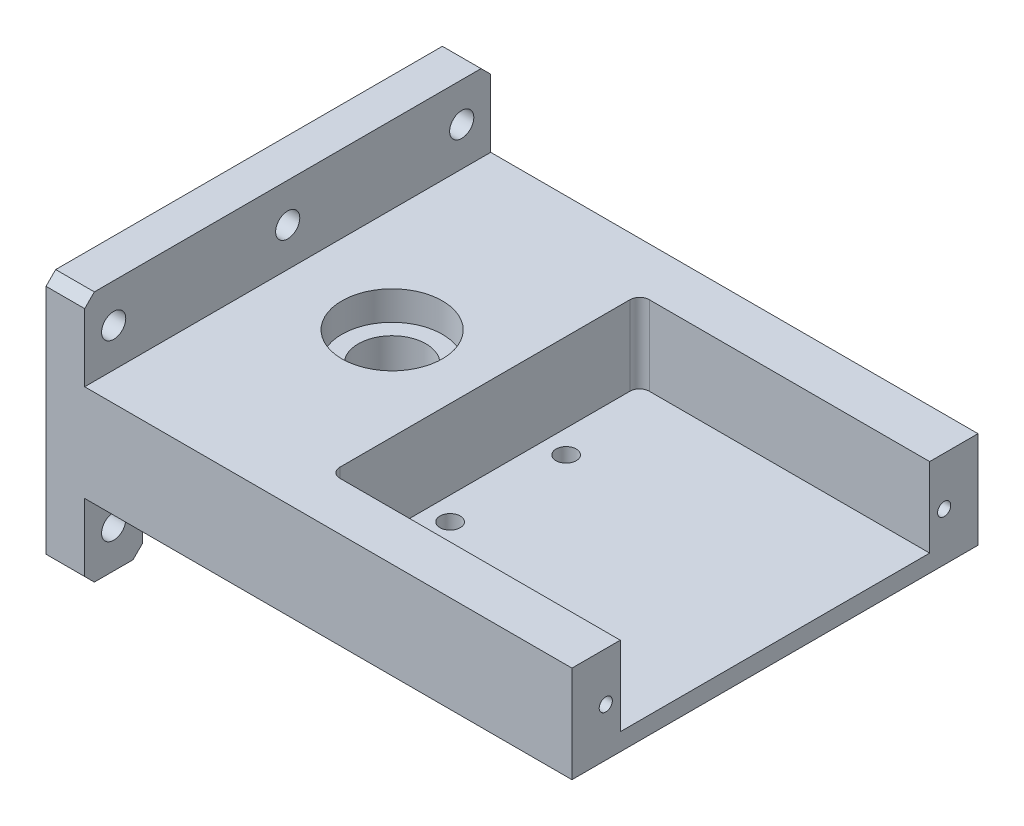
from build123d import *

# Parameters (mm, degrees)
SKETCH_1_W                = 210
SKETCH_1_H                = 130
EXTRUDE_1_DEPTH           = 20
SKETCH_2_W                = 210
SKETCH_2_H                = 50
EXTRUDE_2_DEPTH           = 252
SKETCH_3_R                = 26
CUT_EXTRUDE_1_DEPTH       = 15
SKETCH_4_R                = 17.5
CUT_EXTRUDE_2_DEPTH       = 302.054812285
SKETCH_5_W                = 160
SKETCH_5_H                = 41
CUT_EXTRUDE_3_DEPTH       = 150
HOLE_WIZARD_M8_1_D        = 6.8
HOLE_WIZARD_M8_1_DEPTH    = 19.75
HOLE_WIZARD_M8_1_TIP      = 2.042926105
HOLE_WIZARD_10_5_10_5_1_D = 10.5
SKETCH_10_W               = 150
SKETCH_10_H               = 40
CUT_EXTRUDE_4_DEPTH       = 281.631430884
HOLE_WIZARD_12_5_12_5_1_D = 12.5
CHAMFER_1_SIZE            = 5
FILLET_1_R                = 5


with BuildPart() as part:
    # 草图1 → 凸台-拉伸1 (new body)
    with BuildSketch(Plane(origin=(0, 0, 0), x_dir=(0, 0, -1), z_dir=(1, 0, 0))):
        Rectangle(SKETCH_1_W, SKETCH_1_H)
    extrude(amount=EXTRUDE_1_DEPTH)

    # 草图2 → 凸台-拉伸2 (add)
    with BuildSketch(Plane(origin=(20, 0, 0), x_dir=(0, 0, -1), z_dir=(1, 0, 0))):
        Rectangle(SKETCH_2_W, SKETCH_2_H)
    extrude(amount=EXTRUDE_2_DEPTH)

    # 草图3 → 切除-拉伸1 (cut)
    with BuildSketch(Plane(origin=(0, 25, 0), x_dir=(1, 0, 0), z_dir=(0, 1, 0))):
        with Locations(Location((74, 0, 0), (0, 0, 270))):
            Circle(SKETCH_3_R)
    extrude(amount=-CUT_EXTRUDE_1_DEPTH, mode=Mode.SUBTRACT)

    # 草图4 → 切除-拉伸2 (cut, through all)
    with BuildSketch(Plane(origin=(0, 10, 0), x_dir=(1, 0, 0), z_dir=(0, 1, 0))):
        with Locations(Location((74, 0, 0), (0, 0, 270))):
            Circle(SKETCH_4_R)
    extrude(amount=-CUT_EXTRUDE_2_DEPTH, mode=Mode.SUBTRACT)

    # 草图5 → 切除-拉伸3 (cut)
    with BuildSketch(Plane(origin=(272, 0, 0), x_dir=(0, 0, -1), z_dir=(1, 0, 0))):
        with Locations((0, 4.5)):
            Rectangle(SKETCH_5_W, SKETCH_5_H)
    extrude(amount=-CUT_EXTRUDE_3_DEPTH, mode=Mode.SUBTRACT)

    # M8 螺纹孔1
    with Locations(Plane(origin=(272, 0, 0), x_dir=(0, 0, -1), z_dir=(1, 0, 0))):
        with Locations((-87.5, 0), (87.5, 0)):
            Hole(HOLE_WIZARD_M8_1_D / 2, depth=HOLE_WIZARD_M8_1_DEPTH)
            with Locations((0, 0, -(HOLE_WIZARD_M8_1_DEPTH + HOLE_WIZARD_M8_1_TIP / 2))):  # 118° drill point
                Cone(0, HOLE_WIZARD_M8_1_D / 2, HOLE_WIZARD_M8_1_TIP, mode=Mode.SUBTRACT)

    # Ø10.5 (10.5) 直径孔1 (through all)
    with Locations(Plane(origin=(0, -25, 0), x_dir=(-1, 0, 0), z_dir=(0, -1, 0))):
        with Locations((-134, 30), (-134, -30)):
            Hole(HOLE_WIZARD_10_5_10_5_1_D / 2)

    # 草图10 → 切除-拉伸4 (cut, through all)
    with BuildSketch(Plane(origin=(20, 0, 0), x_dir=(0, 0, -1), z_dir=(1, 0, 0))):
        with Locations((0, -45)):
            Rectangle(SKETCH_10_W, SKETCH_10_H)
    extrude(amount=-CUT_EXTRUDE_4_DEPTH, mode=Mode.SUBTRACT)

    # Ø12.5 (12.5) 直径孔1 (through all)
    with Locations(Plane(origin=(20, 0, 0), x_dir=(0, 0, -1), z_dir=(1, 0, 0))):
        with Locations((-90, 45), (0, 45), (90, 45), (-90, -45), (90, -45)):
            Hole(HOLE_WIZARD_12_5_12_5_1_D / 2)

    # 倒角1
    chamfer_1_edges = [part.edges().sort_by_distance(p)[0] for p in [
        (10, -65, -105),
        (10, -65, 105),
        (10, -65, 75),
        (10, 65, 105),
        (10, -65, -75),
        (10, 65, -105),
    ]]
    chamfer(chamfer_1_edges, length=CHAMFER_1_SIZE)

    # 圆角1
    fillet_1_edges = [part.edges().sort_by_distance(p)[0] for p in [
        (122, 4.5, 80),
        (122, 4.5, -80),
    ]]
    fillet(fillet_1_edges, radius=FILLET_1_R)


solid = part.part
